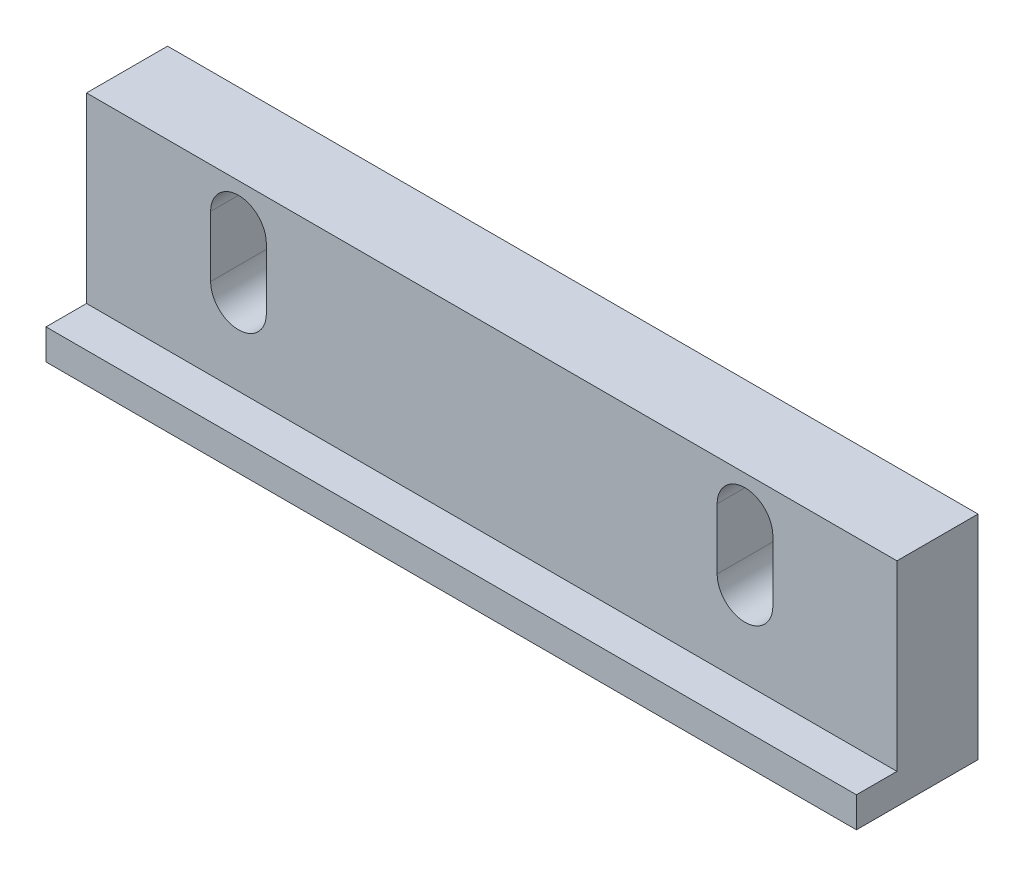
from build123d import *

# Parameters (mm, degrees)
SKETCH_1_W          = 80
SKETCH_1_H          = 21
EXTRUDE_1_DEPTH     = 8
SKETCH_2_W          = 80
SKETCH_2_H          = 3
EXTRUDE_2_DEPTH     = 4
CUT_EXTRUDE_1_DEPTH = 8


with BuildPart() as part:
    # 草图1 → 凸台-拉伸1 (new body)
    with BuildSketch(Plane.XY):
        with Locations((0, 10.5)):
            Rectangle(SKETCH_1_W, SKETCH_1_H)
    extrude(amount=EXTRUDE_1_DEPTH)

    # 草图2 → 凸台-拉伸2 (add)
    with BuildSketch(Plane.XY.offset(8)):
        with Locations((0, 1.5)):
            Rectangle(SKETCH_2_W, SKETCH_2_H)
    extrude(amount=EXTRUDE_2_DEPTH)

    # 草图3 → 切除-拉伸1 (cut)
    with BuildSketch(Plane.XY.offset(8)):
        with BuildLine():
            Line((-22.25, 17), (-22.25, 11))
            ThreePointArc((-22.25, 11), (-25, 8.25), (-27.75, 11))
            Line((-27.75, 11), (-27.75, 17))
            ThreePointArc((-27.75, 17), (-25, 19.75), (-22.25, 17))
        make_face()
    cut_extrude_1 = extrude(amount=-CUT_EXTRUDE_1_DEPTH, mode=Mode.SUBTRACT)

    # 镜向1: 切除-拉伸1 across plane
    add(cut_extrude_1.mirror(Plane.ZY), mode=Mode.SUBTRACT)


solid = part.part
